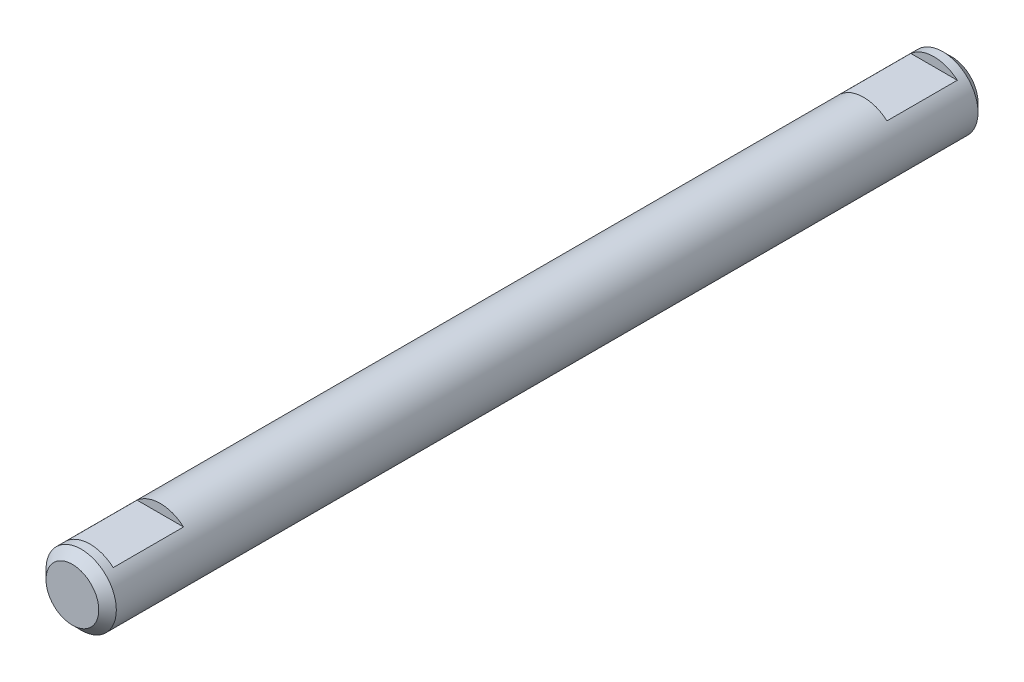
SolidWorks part; units mm, degrees
ref_plane "Front Plane" through (0, 0, 0) normal (0, 0, 1) x (1, 0, 0)
ref_plane "Top Plane" through (0, 0, 0) normal (0, 1, 0) x (1, 0, 0)
ref_plane "Right Plane" through (0, 0, 0) normal (1, 0, 0) x (0, 0, -1)
sketch "Sketch1" plane through (0, 0, 0) normal (0, 0, 1) x (1, 0, 0)
  circle A0 centre (0, 0) radius 2
  dimension "D1" = 4
extrude "Boss-Extrude1" add sketch "Sketch1" along normal mid plane 50
ref_plane "Plane1" through (0, 2, 0) normal (0, 1, 0) x (-1, 0, 0)
sketch "Sketch2" plane through (0, 2, 0) normal (0, 1, 0) x (-1, 0, 0)
  line L0 (-2, -25) -> (2, -25) construction
  line L1 (-7.7093, 24) -> (7.7093, 24)
  line L2 (-7.7093, 24) -> (-7.7093, 20)
  line L3 (-7.7093, 20) -> (7.7093, 20)
  line L4 (7.7093, 24) -> (7.7093, 20)
  line L5 (-5.0318, -20) -> (6.786, -20)
  line L6 (-5.0318, -20) -> (-5.0318, -24)
  line L7 (-5.0318, -24) -> (6.786, -24)
  line L8 (6.786, -20) -> (6.786, -24)
  line L9 (2, 25) -> (-2, 25) construction
  dimension "D1" = 4
  dimension "D2" = 4
  dimension "D3" = 1
  dimension "D4" = 1
extrude "Cut-Extrude1" cut sketch "Sketch2" against normal blind 0.5
chamfer "Chamfer1" distance 0.5 angle 45 2 edges at (2, 0, 25) (2, 0, -25)
